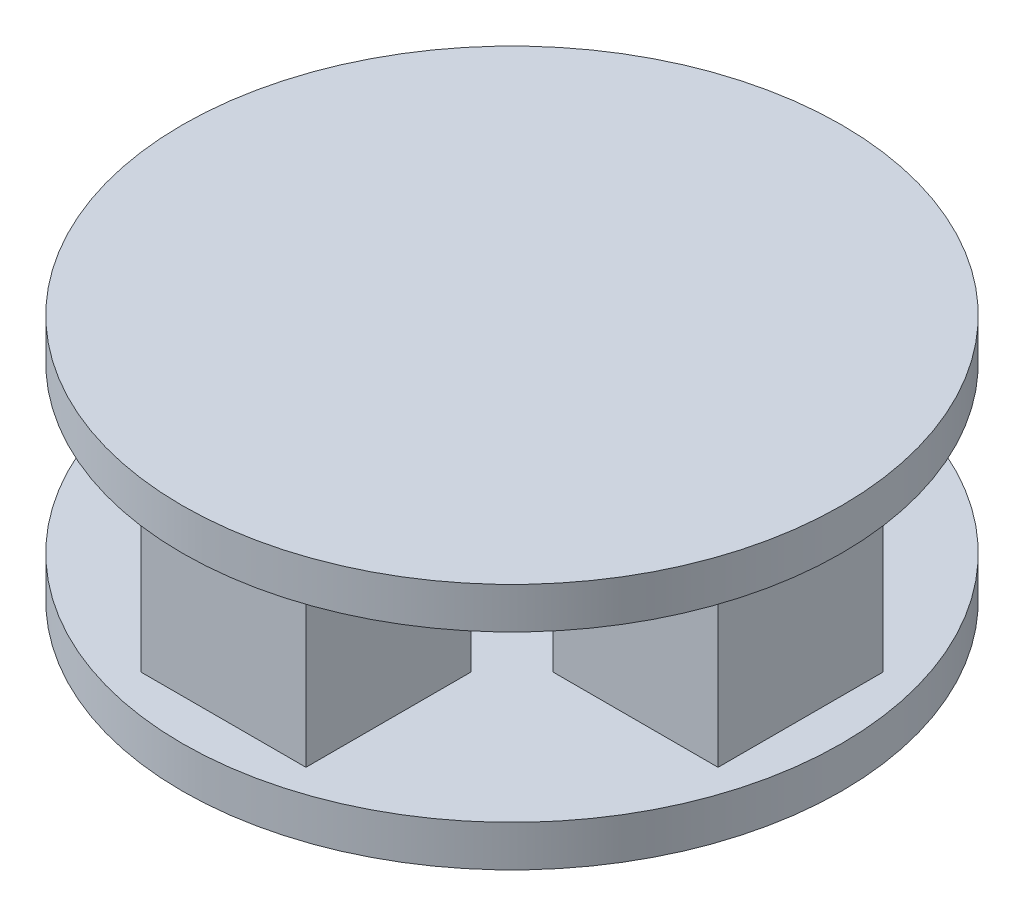
from build123d import *

# Parameters (mm, degrees)
SKETCH1_R           = 16
BOSS_EXTRUDE2_DEPTH = 2
SKETCH4_W           = 8
SKETCH4_H           = 8
BOSS_EXTRUDE7_DEPTH = 8
SKETCH5_R           = 16
BOSS_EXTRUDE8_DEPTH = 2


with BuildPart() as part:
    # Sketch1 → Boss-Extrude2 (new body)
    with BuildSketch(Plane(origin=(0, 0, 0), x_dir=(1, 0, 0), z_dir=(0, 1, 0))):
        with Locations(Location((0, 0, 0), (0, 0, 270))):
            Circle(SKETCH1_R)
    extrude(amount=BOSS_EXTRUDE2_DEPTH)

    # Sketch4 → Boss-Extrude7 (add)
    with BuildSketch(Plane(origin=(0, 2, 0), x_dir=(1, 0, 0), z_dir=(0, 1, 0))):
        with Locations((-10, 0)):
            Rectangle(SKETCH4_W, SKETCH4_H)
        with Locations((0, -10)):
            Rectangle(SKETCH4_W, SKETCH4_H)
        with Locations((0, 10)):
            Rectangle(SKETCH4_W, SKETCH4_H)
        with Locations((10, 0)):
            Rectangle(SKETCH4_W, SKETCH4_H)
    extrude(amount=BOSS_EXTRUDE7_DEPTH)

    # Sketch5 → Boss-Extrude8 (add)
    with BuildSketch(Plane(origin=(0, 10, 0), x_dir=(-1, 0, 0), z_dir=(0, -1, 0))):
        with Locations(Location((0, 0, 0), (0, 0, 270))):
            Circle(SKETCH5_R)
    extrude(amount=-BOSS_EXTRUDE8_DEPTH)


solid = part.part
